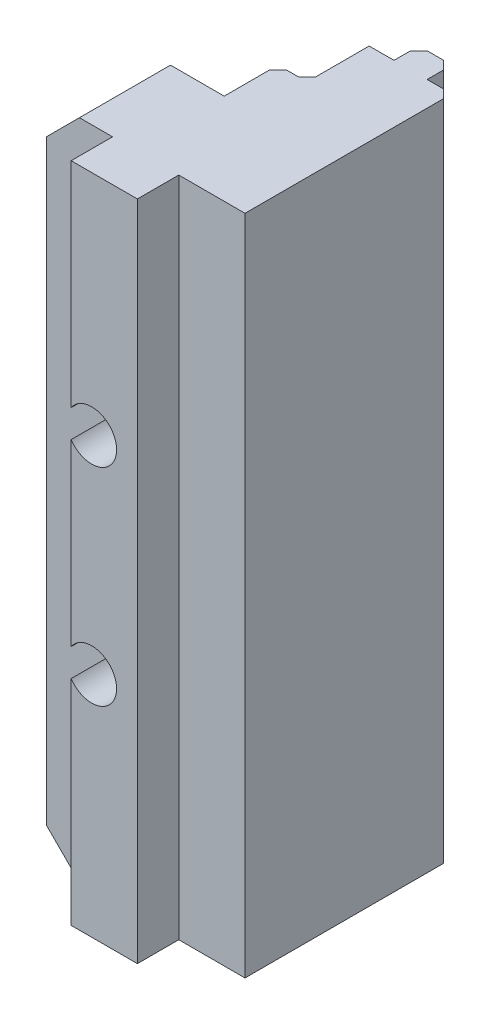
from build123d import *

# Parameters (mm, degrees)
BOSS_EXTRUDE1_DEPTH     = 80
CHAMFER1_SIZE           = 1
CHAMFER2_SIZE           = 4
SKETCH2_W               = 8
SKETCH2_H               = 5
BOSS_EXTRUDE2_DEPTH     = 80
SKETCH3_R               = 4
CUT_EXTRUDE1_DEPTH      = 7.5
CUT_EXTRUDE2_DEPTH      = 86.234969349
CUT_EXTRUDE2_DEPTH_BACK = 86.234969349
SKETCH4_R               = 3
CUT_EXTRUDE3_DEPTH      = 89.090862182
CUT_EXTRUDE3_DEPTH_BACK = 3
SKETCH5_R               = 1.5


with BuildPart() as part:
    # Sketch1 → Boss-Extrude1 (new body)
    with BuildSketch(Plane(origin=(0, 0, 0), x_dir=(1, 0, 0), z_dir=(0, 1, 0))):
        Polygon((0, 25), (0, 0), (-24, 0), (-24, 7.06470747), (-20.721166606, 11), (-13.511532016, 11), (-13.511532016, 17.5), (-10, 17.5), (-10, 25), (-7, 25), (-7, 28), (-3, 28), (-3, 25), align=None)
    extrude(amount=BOSS_EXTRUDE1_DEPTH)

    # Chamfer1
    chamfer1_edges = [part.edges().sort_by_distance(p)[0] for p in [
        (-13.511532016, 40, -17.5),
        (-10, 40, -17.5),
        (-7, 40, -28),
        (-3, 40, -28),
        (0, 40, -25),
    ]]
    chamfer(chamfer1_edges, length=CHAMFER1_SIZE)

    # Chamfer2
    chamfer2_edges = [part.edges().sort_by_distance(p)[0] for p in [
        (-24, 80, -3.532353735),
        (-24, 0, -3.532353735),
    ]]
    chamfer(chamfer2_edges, length=CHAMFER2_SIZE)

    # Sketch2 → Boss-Extrude2 (add)
    with BuildSketch(Plane(origin=(0, 80, 0), x_dir=(1, 0, 0), z_dir=(0, 1, 0))):
        with Locations((-12, -2.5)):
            Rectangle(SKETCH2_W, SKETCH2_H)
    extrude(amount=-BOSS_EXTRUDE2_DEPTH)

    # Sketch3 → Cut-Extrude1 (cut, symmetric)
    with BuildSketch(Plane(origin=(0, 0, -11), x_dir=(-1, 0, 0), z_dir=(0, 0, -1))):
        with Locations((13.511532016, 52.5)):
            Circle(SKETCH3_R)
        with Locations(Location((13.511532016, 27.5, 0), (0, 0, 90))):
            Circle(SKETCH3_R)
    extrude(amount=CUT_EXTRUDE1_DEPTH, both=True, mode=Mode.SUBTRACT)

    # Sketch4 → Cut-Extrude2 (cut, two sides: drawn at the far end of the back side and taken through both)
    with BuildSketch(Plane(origin=(0, 0, -11), x_dir=(-1, 0, 0), z_dir=(0, 0, -1)).offset(-CUT_EXTRUDE2_DEPTH_BACK)):
        with Locations((13.511532016, 52.5)):
            Circle(SKETCH4_R)
        with Locations(Location((13.511532016, 27.5, 0), (0, 0, 33.953684666))):
            Circle(SKETCH4_R)
    extrude(amount=CUT_EXTRUDE2_DEPTH + CUT_EXTRUDE2_DEPTH_BACK, mode=Mode.SUBTRACT)

    # Sketch5 → Cut-Extrude3 (cut, two sides: drawn at the far end of the back side and taken through both)
    with BuildSketch(Plane.XY.offset(-CUT_EXTRUDE3_DEPTH_BACK)):
        with Locations(Location((-19, 40, 0), (0, 0, 180))):
            Circle(SKETCH5_R)
    extrude(amount=CUT_EXTRUDE3_DEPTH + CUT_EXTRUDE3_DEPTH_BACK, mode=Mode.SUBTRACT)


solid = part.part
